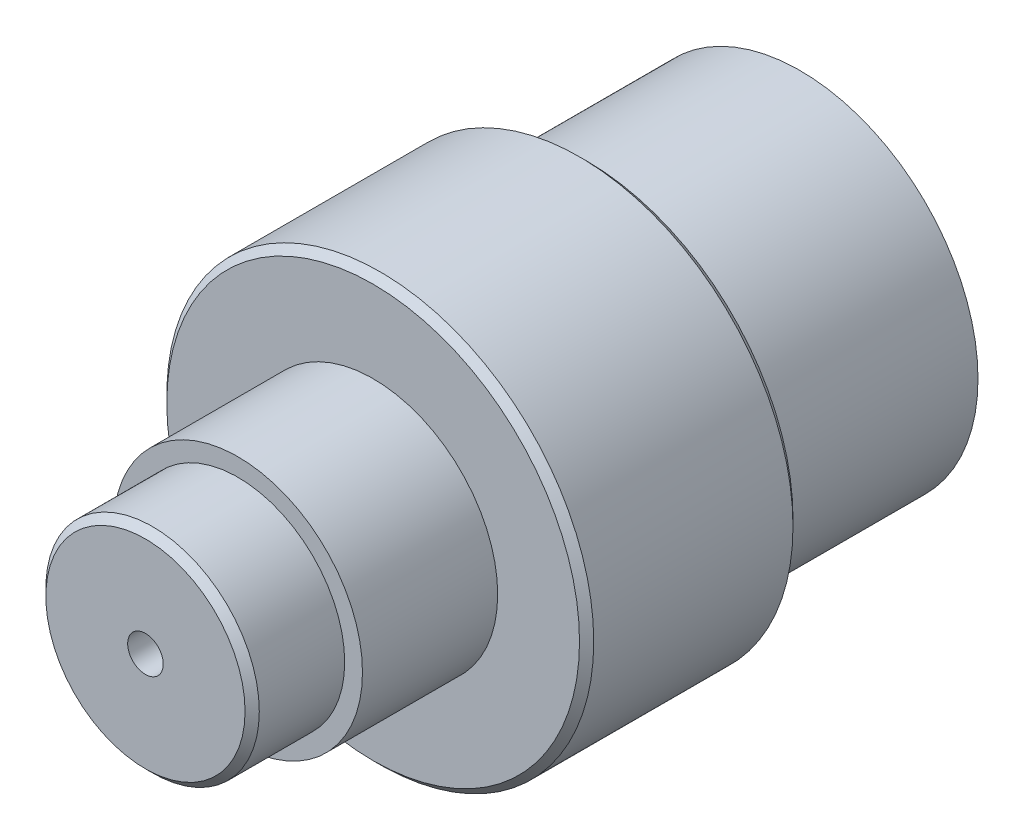
SolidWorks part; units mm, degrees
material "Q235A"
ref_plane "前视基准面" through (0, 0, 0) normal (0, 0, 1) x (1, 0, 0)
ref_plane "上视基准面" through (0, 0, 0) normal (0, 1, 0) x (1, 0, 0)
ref_plane "右视基准面" through (0, 0, 0) normal (1, 0, 0) x (0, 0, -1)
sketch "草图1" plane through (0, 0, 0) normal (0, 0, 1) x (1, 0, 0)
  circle A0 centre (0, 0) radius 25
  dimension "D1" = 50
extrude "凸台-拉伸1" add sketch "草图1" along normal blind 30
sketch "草图2" plane through (0, 0, 30) normal (0, 0, 1) x (1, 0, 0)
  circle A0 centre (0, 0) radius 30
  dimension "D1" = 60
extrude "凸台-拉伸2" add sketch "草图2" along normal blind 30
sketch "草图4" plane through (0, 0, 0) normal (0, 0, -1) x (-1, 0, 0)
  circle A0 centre (0, 0) radius 15
  dimension "D1" = 30
extrude "切除-拉伸1" cut sketch "草图4" against normal through all
sketch "草图6" plane through (0, 0, 60) normal (0, 0, 1) x (1, 0, 0)
  line L0 (0, 30) -> (0, 0) construction
  line L1 (-13.0767, 27) -> (13.0767, 27)
  line L2 (27, 13.0767) -> (27, -13.0767)
  line L3 (13.0767, -27) -> (-13.0767, -27)
  line L4 (-27, -13.0767) -> (-27, 13.0767)
  line L5 (0, 0) -> (13.0767, 27) construction
  arc A0 (27, -13.0767) -> (27, 13.0767) centre (0, 0) ccw
  circle A1 centre (0, 0) radius 30
  arc A2 (13.0767, 27) -> (-13.0767, 27) centre (0, 0) ccw
  arc A3 (-13.0767, -27) -> (13.0767, -27) centre (0, 0) ccw
  arc A4 (-27, 13.0767) -> (-27, -13.0767) centre (0, 0) ccw
  dimension "D2" = 3
  dimension "D1" = 0
  dimension "D3" = 4
extrude "切除-拉伸2" [suppressed] cut sketch "草图6" against normal offset from surface (25 mm away) 5
sketch "草图13" plane through (0, 0, 60) normal (0, 0, 1) x (1, 0, 0)
  circle A0 centre (0, 0) radius 15 construction
  circle A1 centre (0, 0) radius 15
extrude "凸台-拉伸4" add sketch "草图13" against normal offset from surface (30 mm away) 30 up to face at (-15, 0, 0)
sketch "草图12" plane through (0, 0, 60) normal (0, 0, 1) x (1, 0, 0)
  circle A0 centre (0, 0) radius 17.5
  dimension "D1" = 35
extrude "凸台-拉伸3" add sketch "草图12" along normal blind 32
hole_wizard "M6 螺纹孔1" positions "草图14" profile "草图15" tap size "M6" standard "ISO"
sketch "草图14" plane through (0, 0, 92) normal (0, 0, 1) x (1, 0, 0)
  point P0 (0, 0)
sketch "草图15" plane through (0, 0, 92) normal (1, 0, 0) x (0, -1, 0)
  line L0 (0, 0) -> (0, 16.5022)
  line L1 (0, 16.5022) -> (2.5, 15)
  line L2 (2.5, 15) -> (2.5, 0)
  line L5 (2.5, 0) -> (0, 0)
  line L10 (0, 16.5022) -> (-2.5, 15) construction
  line L11 (0, -6.35) -> (0, 107.95) construction
  dimension "螺纹孔钻头直径" = 5
  dimension "螺纹孔钻头深度" = 15
  dimension "导头角度" = 118
cosmetic thread "孔螺蚊线1" parameters "D1"=12, "D2"=6
sketch "草图16" plane through (0, 0, 92) normal (0, 0, 1) x (1, 0, 0)
  circle A0 centre (0, 0) radius 15
  circle A1 centre (0, 0) radius 17.5
  circle A2 centre (0, 0) radius 17.5
  dimension "D2" = 30
  dimension "D1" = 0
extrude "切除-拉伸3" cut sketch "草图16" against normal blind 13
chamfer "倒角4" distance 1 angle 45 4 edges at (-15, 0, 0) (15, 0, 92) (30, 0, 30) (30, 0, 60)
